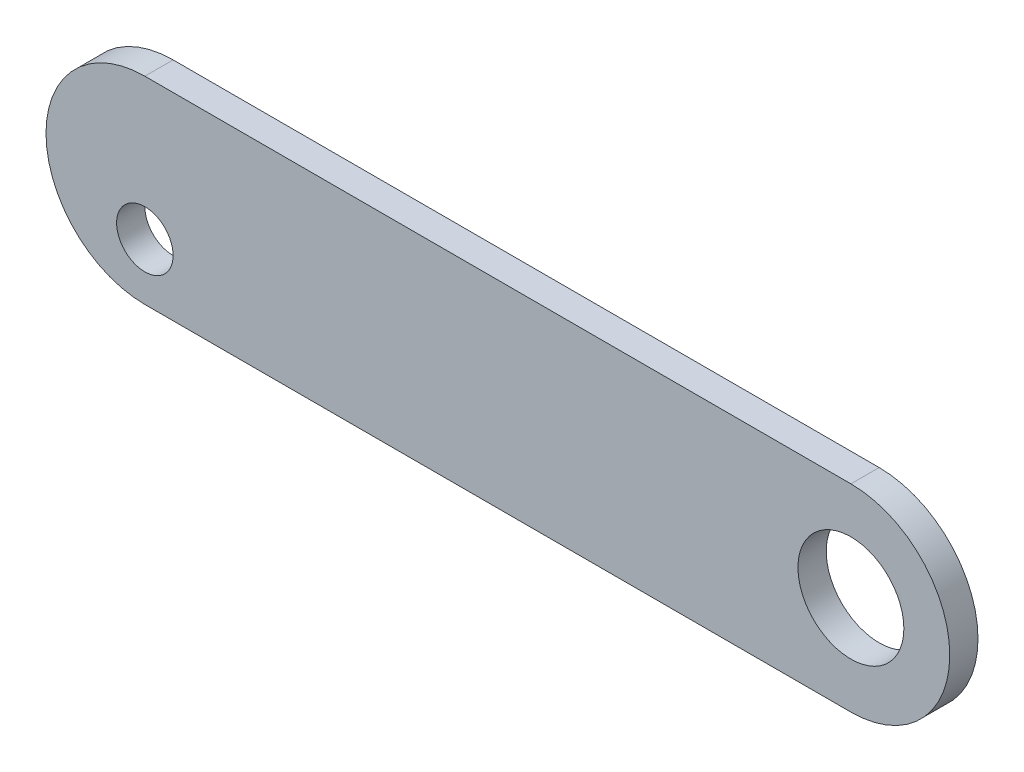
from build123d import *

# Parameters (mm, degrees)
SKETCH_1_R      = 37.5
SKETCH_1_R_2    = 20
EXTRUDE_1_DEPTH = 20


with BuildPart() as part:
    # 草图1 → 凸台-拉伸1 (new body)
    with BuildSketch(Plane.XY):
        with BuildLine():
            Line((-250, 70), (250, 70))
            ThreePointArc((250, 70), (320, 0), (250, -70))
            Line((250, -70), (-250, -70))
            ThreePointArc((-250, -70), (-320, 0), (-250, 70))
        make_face()
        with Locations((250, 0)):
            Circle(SKETCH_1_R, mode=Mode.SUBTRACT)
        with Locations((-250, -30)):
            Circle(SKETCH_1_R_2, mode=Mode.SUBTRACT)
    extrude(amount=EXTRUDE_1_DEPTH)


solid = part.part
